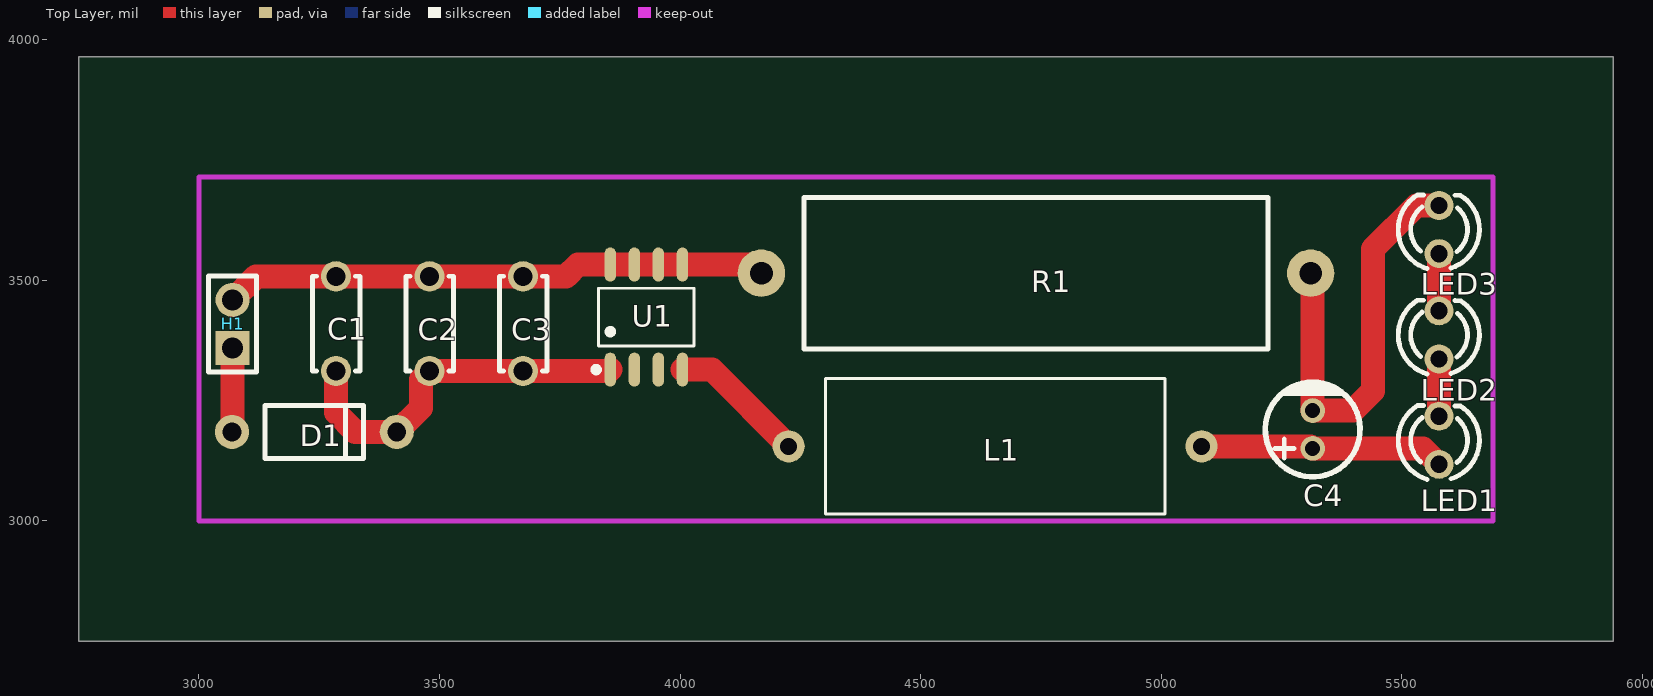
[diagram p0: Top Layer view]
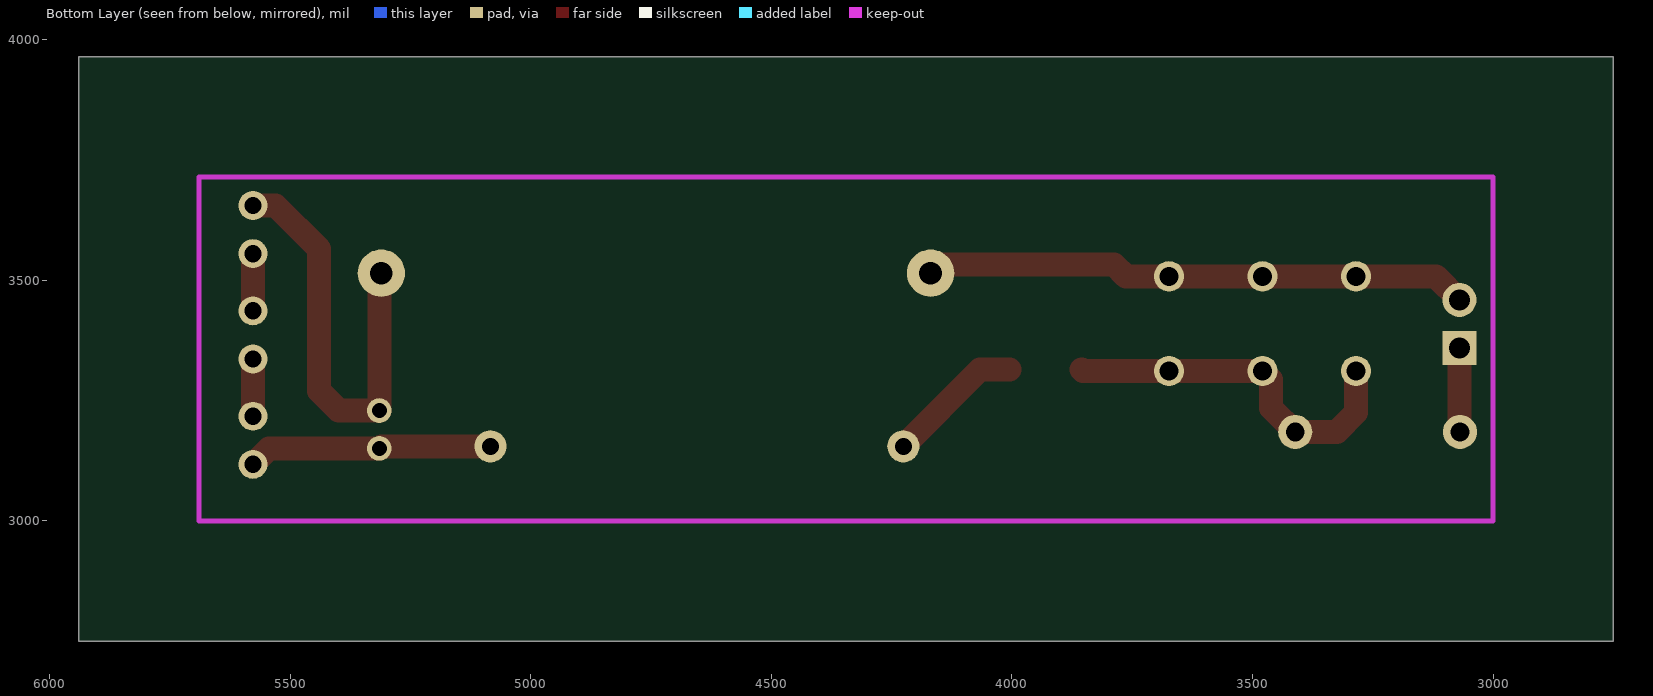
[diagram p1: Bottom Layer view, seen from below]
# Altium PCB MISC51773.pcbdoc
Units mil, origin at the board's own origin, x right, y up, seen from the top; angles counter-clockwise.
Board outline 3190 x 1215 mil, 2 copper layers (Top Layer, Bottom Layer), stack 62.206 mil thick; 12 components, 8 nets, 30 pads, 0 vias.

## Layer stack, top to bottom
Top Solder Mask Layer: solder mask 0.394, Dk 3.3
Top Layer: signal copper 1.379
Dielectric1: surface 59.449, FR4, Dk 4.5
Bottom Layer: signal copper 1.378
Bottom Solder Mask Layer: solder mask 0.394, Dk 3.3

## Board outline
5940,2750 2750,2750 2750,3965 5940,3965

## Design rules (kind name [scope] priority, off if disabled: settings)
BoardOutlineClearance copperThickness2oz_1 [All] p2 off: genericclearance=7.99 ignorepadtopadclearanceinfootprint=FALSE except(0: Arc-SplitContinuation Track-SplitContinuation SMDPad-SplitContinuation THPad-SplitContinuation Via-SplitContinuation Fill-SplitContinuation Region-SplitContinuation Poly-SplitContinuation Text-SplitContinuation Hole-SplitContinuation; 5.98: Arc-CutoutEdge SMDPad-CutoutEdge THPad-CutoutEdge Via-CutoutEdge Fill-CutoutEdge Region-CutoutEdge Text-CutoutEdge; 6.93: Hole-OutlineEdge Hole-CutoutEdge; 10: Poly-OutlineEdge Poly-CutoutEdge; 11.81: Arc-OutlineEdge Track-OutlineEdge SMDPad-OutlineEdge THPad-OutlineEdge Via-OutlineEdge Fill-OutlineEdge Region-OutlineEdge Text-OutlineEdge Track-CutoutEdge)
BoardOutlineClearance copperThickness1oz_1 [All] p4: genericclearance=4.02 ignorepadtopadclearanceinfootprint=FALSE except(0: Arc-SplitContinuation Track-SplitContinuation SMDPad-SplitContinuation THPad-SplitContinuation Via-SplitContinuation Fill-SplitContinuation Region-SplitContinuation Poly-SplitContinuation Text-SplitContinuation Hole-SplitContinuation; 6: SMDPad-CutoutEdge THPad-CutoutEdge Via-CutoutEdge Fill-CutoutEdge Region-CutoutEdge Text-CutoutEdge; 6.93: Hole-OutlineEdge Hole-CutoutEdge; 10: Poly-OutlineEdge Poly-CutoutEdge; 11.8: Arc-OutlineEdge Track-OutlineEdge SMDPad-OutlineEdge THPad-OutlineEdge Via-OutlineEdge Fill-OutlineEdge Region-OutlineEdge Text-OutlineEdge; 11.81: Arc-CutoutEdge Track-CutoutEdge)
Clearance copperThickness2oz [All] p1 off: gap=7.99 ignorepadtopadclearanceinfootprint=FALSE except(5.98: SMDPad-Track SMDPad-SMDPad THPad-Track SMDPad-THPad THPad-THPad Track-Via SMDPad-Via THPad-Via Via-Via Fill-Track Region-Track Fill-SMDPad Region-SMDPad Fill-THPad Region-THPad Fill-Via Region-Via Fill-Fill Fill-Region Region-Region Arc-Track Arc-SMDPad Arc-THPad Arc-Via Fill-Arc Region-Arc Arc-Arc Text-Track SMDPad-Text Text-THPad Text-Via Fill-Text Region-Text Arc-Text Text-Text; 6.93: Hole-Track Hole-SMDPad Hole-THPad Hole-Via Fill-Hole Region-Hole Hole-Arc Hole-Text; 10: Poly-Track Poly-SMDPad Poly-THPad Poly-Via Poly-Fill Poly-Region Poly-Poly Poly-Arc Poly-Text Poly-Hole)
Clearance copperThickness1oz [All] p3: gap=4.02 ignorepadtopadclearanceinfootprint=FALSE except(5.98: SMDPad-Track SMDPad-SMDPad THPad-Track SMDPad-THPad THPad-THPad Track-Via SMDPad-Via THPad-Via Via-Via Fill-Track Region-Track Fill-SMDPad Region-SMDPad Fill-THPad Region-THPad Fill-Via Region-Via Fill-Fill Fill-Region Region-Region; 6: Arc-Track Arc-SMDPad Arc-THPad Arc-Via Fill-Arc Region-Arc Arc-Arc Text-Track SMDPad-Text Text-THPad Text-Via Fill-Text Region-Text Arc-Text Text-Text; 6.93: Hole-Track Hole-SMDPad Hole-THPad Hole-Via Fill-Hole Region-Hole Hole-Arc Hole-Text; 10: Poly-Track Poly-SMDPad Poly-THPad Poly-Via Poly-Fill Poly-Region Poly-Poly Poly-Arc Poly-Text Poly-Hole)
DiffPairsRouting differentialPair [All] p1: maxlimit=6 minlimit=6 mostfreqgap=6 toplayer_minwidth=5 toplayer_prefwidth=10 toplayer_maxwidth=100 toplayer_mingap=6 toplayer_prefgap=6 toplayer_maxgap=6 bottomlayer_minwidth=5 bottomlayer_prefwidth=10 bottomlayer_maxwidth=100 bottomlayer_mingap=6 bottomlayer_prefgap=6 bottomlayer_maxgap=6 maxuncoupledlength=10
HoleToHoleClearance otherClearance [All] p1: gap=11.81 allowstackedmicrovias=TRUE
Length netLength [All] p1: minlimit=0 maxlimit=0
MatchedLengths netLengthTolerance [All] p1: tolerance=1000
PasteMaskExpansion pasteMaskExpansion [All] p1: expansion=0
PlaneConnect innerPlane [All] p1: planeconnectstyle=Relief reliefexpansion=20 reliefentries=4 reliefconductorwidth=10 reliefairgap=10
PolygonConnect copperRegion [All] p1: connectstyle=Relief reliefconductorwidth=10 reliefentries=4 polygonreliefangle="90 Angle" airgapwidth=10 via.connectstyle=Relief via.reliefconductorwidth=10 via.reliefentries=4 via.polygonreliefangle="90 Angle" via.airgapwidth=10
RoutingVias viaSize [All] p1: holewidth=12.01 width=24.02 viastyle="Through Hole" minholewidth=11.81 minwidth=19.68 maxholewidth=248.03 maxwidth=393.7
SolderMaskExpansion solderMaskExpansion [IsVia] p1: expansion=-1000 istentingtop=TRUE
SolderMaskExpansion solderMaskExpansion [All] p2: expansion=2 istentingtop=FALSE
Width copperThickness2oz_2 [All] p1 off: maxlimit=100 minlimit=8 preferedwidth=10
Width copperThickness1oz_2 [All] p2: maxlimit=100 minlimit=5 preferedwidth=10

## Components (designator, comment, footprint, x,y, rotation, side; value= is the part's Value field where it differs from the comment)
C1 "100nF" CAP-TH_L5.0-W2.5-P5.00-D1.0 3285,3410 r90 top
C2 "100nF" CAP-TH_L5.0-W2.5-P5.00-D1.0 3479.34,3410 r90 top
C3 "10nF" CAP-TH_L5.0-W2.5-P5.00-D1.0 3673.67,3410 r90 top
C4 "10uF" CAP-TH_BD5.0-P2.00-D0.8-FD-10UF50VC110GL 5315,3190 r90 top
D1 "" DO_1N4007 3240,3185 r180 top
H1 "" HDR-TH_2P-P2.54-V-M-1 3070,3409.35 r90 top
L1 "47uH" IND-TH_BD7.0-L17.8-P21.80-D0.8 4655,3155 r0 top
LED1 "" LED_TH-3mm 5577.71,3167.54 r90 top
LED2 "" LED_TH-3mm 5577.71,3386.58 r90 top
LED3 "" LED_TH-3mm 5577.71,3605.62 r90 top
R1 "0.68Ω" Res_5W 4740,3510 r0 top
U1 "PT4501C" SOP-8_L4.9-W3.9-P1.27-LS6.0-BL-EP 3930,3423.62 r0 top

## Footprints (in the part's own frame and the unit in brackets; to place one, negate y for a bottom-side part, rotate by r counter-clockwise, add the part's x,y. Pads: shape width x height; smd on the part's side, far side on the other; paste and mask are expansions set on the pad)
CAP-TH_BD5.0-P2.00-D0.8-FD-10UF50VC110GL [mm]
  round 1.3 hole 0.8: 1(-1,0) 2(1,0)
  silkscreen extent -2.5,-2.5 2.5,2.5
CAP-TH_L5.0-W2.5-P5.00-D1.0 [mm]
  round 1.6 hole 1: 1(-2.5,0) 2(2.5,0)
  silkscreen extent -2.5,-1.27 2.5,1.25
DO_1N4007 [mm]
  round 1.8 hole 1 paste+0 mask+0.051: 1(-4.35,0) 2(4.35,0)
  silkscreen extent -2.6,-1.4 2.6,1.4
HDR-TH_2P-P2.54-V-M-1 [mm]
  rect 1.8x1.8 hole 1.1: 1(-1.27,0)
  round 1.8 hole 1.1: 2(1.27,0)
  silkscreen extent -2.54,-1.27 2.54,1.27
IND-TH_BD7.0-L17.8-P21.80-D0.8 [mm]
  round 1.7 hole 0.9: 1(-10.9,0) 2(10.9,0)
  silkscreen extent -8.97,-3.58 8.97,3.58
LED_TH-3mm [mil]
  round 60 hole 36 paste+0 mask+2: 1(-50,0) 2(50,0)
  silkscreen extent -81,-84 72,85
Res_5W [mm]
  round 2.5 hole 1.2 paste+0 mask+0.051: 1(-14.5,0.127) 2(14.5,0.127)
  silkscreen extent -12.25,-3.87 12.25,4.13
SOP-8_L4.9-W3.9-P1.27-LS6.0-BL-EP [mm]
  oval 0.6x1.8 smd: 1(-1.905,-2.772) 2(-0.635,-2.772) 3(0.635,-2.772) 4(1.905,-2.772) 5(1.905,2.772) 6(0.635,2.772) 7(-0.635,2.772) 8(-1.905,2.772)
  silkscreen extent -2.8,-2.92 2.53,1.52

## Nets (pads, with @x,y where several pads share a name; then routed paths per layer and width w, separated by ;. In a path a pad name is that pad's centre, name@x,y a point inside that pad or via, vN(x,y) a via of type N, cw(c..) or ccw(c..) an arc to the next point about the centre after c; other vN are vias at no path point)
$1N2: C1.1 C2.1 C3.1 D1.1 U1.1 | length 761
  Top Layer w50: C1.1 3285,3225 3325,3185 D1.1 3461.26,3235 3461.26,3293.5 C2.1 C3.1 3852.11,3311.57 U1.1
$1N3: D1.2 H1.1 | length 174.9
  Top Layer w50: D1.2 3070,3186.26 H1.1
$1N5: L1.1 U1.4 | length 286.9
  Top Layer w50: U1.4 4066.4,3314.47 L1.1
$1N6: C4.1 L1.2 LED1.1 | length 509.1
  Top Layer w50: L1.2 5310.63,3155 C4.1 5544.62,3150.63 LED1.1
$1N7: C4.2 LED3.2 R1.2 | length 899.4
  Top Layer w50: R1.2 5315,3510.87 C4.2 5399.37,3229.37 5440,3270 5440,3565 5530.62,3655.62 LED3.2
$1N9: LED1.2 LED2.1 | length 119
  Top Layer w50: LED1.2 LED2.1
$1N10: LED2.2 LED3.1 | length 119
  Top Layer w50: LED2.2 LED3.1
GND: C1.2 C2.2 C3.2 H1.2 R1.1 U1.5 U1.6 U1.7 U1.8 | length 1136.9
  Top Layer w50: H1.2 3119.07,3508.43 C1.2 C2.2 C3.2 3763.43,3508.43 3787.77,3532.77 U1.8 U1.7 U1.6 U1.5 4151.36,3532.77 R1.1
pads on no net: U1.2 U1.3

## Keep-outs
Board Outline Layer:
  lines w10: 3000,3000 3000,3715 5690,3715 5690,3000 3000,3000